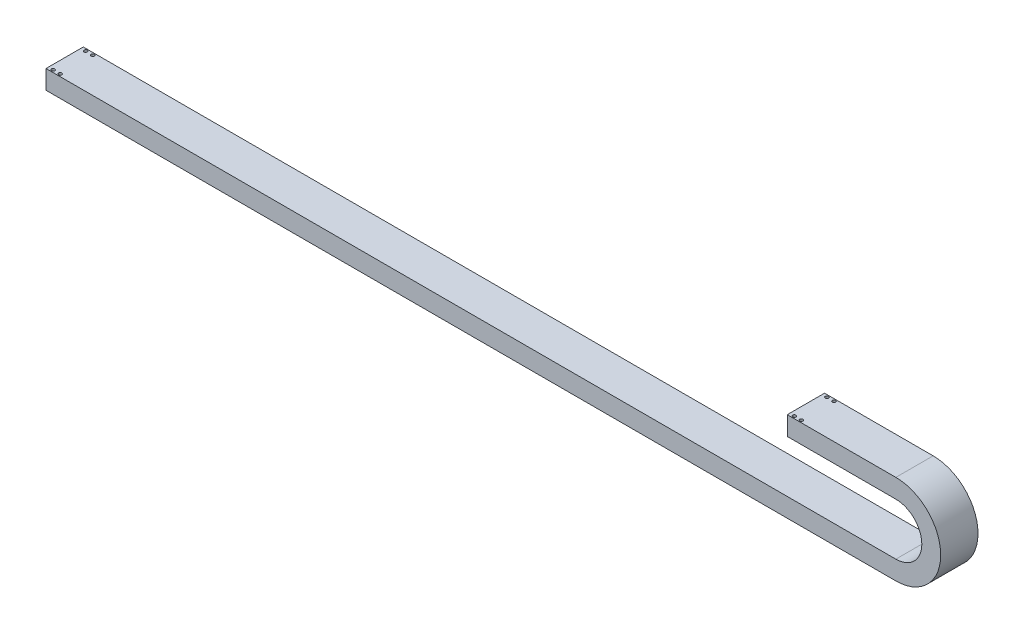
from build123d import *

# Parameters (mm, degrees)
EXTRUDE_1_DEPTH           = 79
HOLE_WIZARD_7_0_7_1_D     = 7
HOLE_WIZARD_7_0_7_2_D     = 7
HOLE_WIZARD_7_0_7_2_DEPTH = 40


with BuildPart() as part:
    # 草图1 → 凸台-拉伸1 (new body)
    with BuildSketch(Plane.XY):
        with BuildLine():
            Line((-327.90073838, 19.409448819), (-97.90073838, 19.409448819))
            ThreePointArc((-97.90073838, 19.409448819), (-42.90073838, -35.590551181), (-97.90073838, -90.590551181))
            Line((-97.90073838, -90.590551181), (-1897.90073838, -90.590551181))
            Line((-1897.90073838, -90.590551181), (-1897.90073838, -130.590551181))
            Line((-1897.90073838, -130.590551181), (-97.90073838, -130.590551181))
            ThreePointArc((-97.90073838, -130.590551181), (-2.90073838, -35.590551181), (-97.90073838, 59.409448819))
            Line((-97.90073838, 59.409448819), (-327.90073838, 59.409448819))
            Line((-327.90073838, 59.409448819), (-327.90073838, 19.409448819))
        make_face()
    extrude(amount=EXTRUDE_1_DEPTH)

    # Ø7.0 (7) 直径孔1 (through all)
    with Locations(Plane(origin=(0, -130.590551181, 0), x_dir=(-1, 0, 0), z_dir=(0, -1, 0))):
        with Locations((1872.90073838, -5), (1887.90073838, -5), (1872.90073838, -74), (1887.90073838, -74)):
            Hole(HOLE_WIZARD_7_0_7_1_D / 2)

    # Ø7.0 (7) 直径孔2
    with Locations(Plane(origin=(0, 59.409448819, 0), x_dir=(1, 0, 0), z_dir=(0, 1, 0))):
        with Locations((-317.90073838, -5), (-302.90073838, -5), (-317.90073838, -74), (-302.90073838, -74)):
            Hole(HOLE_WIZARD_7_0_7_2_D / 2, depth=HOLE_WIZARD_7_0_7_2_DEPTH)


solid = part.part
